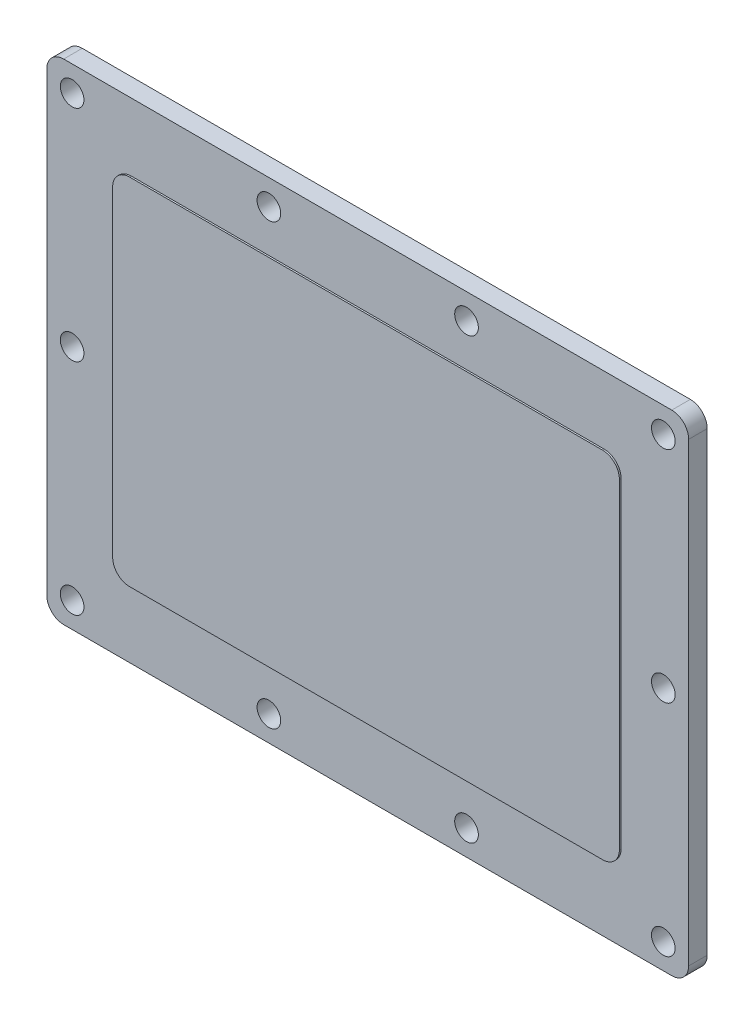
from build123d import *

# Parameters (mm, degrees)
SKETCH1_R           = 7
BOSS_EXTRUDE1_DEPTH = 12
SKETCH2_OUTSIDE_W   = 477.634
SKETCH2_OUTSIDE_H   = 387.634
CUT_EXTRUDE1_DEPTH  = 1


with BuildPart() as part:
    # Sketch1 → Boss-Extrude1 (new body)
    with BuildSketch(Plane.XY):
        with BuildLine():
            Line((10, 0), (370, 0))
            ThreePointArc((370, 0), (377.071067812, 2.928932188), (380, 10))
            Line((380, 10), (380, 280))
            ThreePointArc((380, 280), (377.071067812, 287.071067812), (370, 290))
            Line((370, 290), (10, 290))
            ThreePointArc((10, 290), (2.928932188, 287.071067812), (0, 280))
            Line((0, 280), (0, 10))
            ThreePointArc((0, 10), (2.928932188, 2.928932188), (10, 0))
        make_face()
        with Locations((15, 275)):
            Circle(SKETCH1_R, mode=Mode.SUBTRACT)
        with Locations((131.5, 275)):
            Circle(SKETCH1_R, mode=Mode.SUBTRACT)
        with Locations((248.5, 275)):
            Circle(SKETCH1_R, mode=Mode.SUBTRACT)
        with Locations((365, 275)):
            Circle(SKETCH1_R, mode=Mode.SUBTRACT)
        with Locations((365, 145)):
            Circle(SKETCH1_R, mode=Mode.SUBTRACT)
        with Locations((365, 15)):
            Circle(SKETCH1_R, mode=Mode.SUBTRACT)
        with Locations((248.5, 15)):
            Circle(SKETCH1_R, mode=Mode.SUBTRACT)
        with Locations((131.5, 15)):
            Circle(SKETCH1_R, mode=Mode.SUBTRACT)
        with Locations((15, 15)):
            Circle(SKETCH1_R, mode=Mode.SUBTRACT)
        with Locations((15, 145)):
            Circle(SKETCH1_R, mode=Mode.SUBTRACT)
    extrude(amount=BOSS_EXTRUDE1_DEPTH)

    # Sketch2 outside → Cut-Extrude1 (cut)
    with BuildSketch(Plane.XY.offset(12)):
        with Locations((190, 145)):
            Rectangle(SKETCH2_OUTSIDE_W, SKETCH2_OUTSIDE_H)
        with BuildLine():
            Line((50, 250), (330, 250))
            ThreePointArc((330, 250), (337.071067812, 247.071067812), (340, 240))
            Line((340, 240), (340, 50))
            ThreePointArc((340, 50), (337.071067812, 42.928932188), (330, 40))
            Line((330, 40), (50, 40))
            ThreePointArc((50, 40), (42.928932188, 42.928932188), (40, 50))
            Line((40, 50), (40, 240))
            ThreePointArc((40, 240), (42.928932188, 247.071067812), (50, 250))
        make_face(mode=Mode.SUBTRACT)
    extrude(amount=-CUT_EXTRUDE1_DEPTH, mode=Mode.SUBTRACT)


solid = part.part
